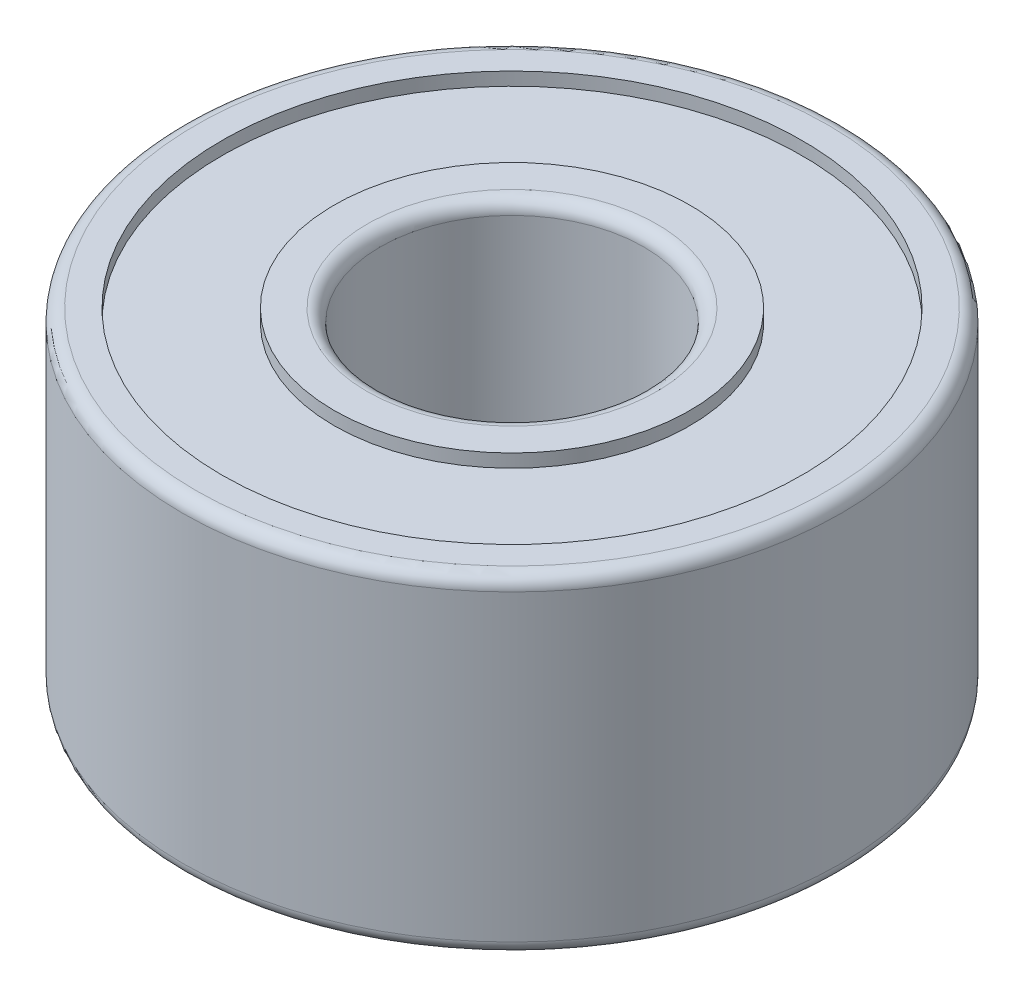
SolidWorks part; units mm, degrees
material "镀铬不锈钢"
ref_plane "前视基准面" through (0, 0, 0) normal (0, 0, 1) x (1, 0, 0)
ref_plane "上视基准面" through (0, 0, 0) normal (0, 1, 0) x (1, 0, 0)
ref_plane "右视基准面" through (0, 0, 0) normal (1, 0, 0) x (0, 0, -1)
sketch "草图1" plane through (0, 0, 0) normal (0, 1, 0) x (1, 0, 0)
  circle A0 centre (0, 0) radius 2.5
  circle A1 centre (0, 0) radius 1
  dimension "D1" = 5
  dimension "D2" = 2
extrude "凸台-拉伸1" add sketch "草图1" along normal blind 2.5
sketch "草图2" plane through (0, 2.5, 0) normal (0, 1, 0) x (1, 0, 0)
  circle A0 centre (0, 0) radius 2.2
  circle A1 centre (0, 0) radius 1.35
  dimension "D1" = 4.4
  dimension "D2" = 2.7
extrude "切除-拉伸1" cut sketch "草图2" against normal blind 0.1
sketch "草图4" plane through (0, 0, 0) normal (0, -1, 0) x (1, 0, 0)
  circle A1 centre (0, 0) radius 1.35
  circle A2 centre (0, 0) radius 1.35
  circle A3 centre (0, 0) radius 2.2
  circle A4 centre (0, 0) radius 2.2
  dimension "D1" = 0
  dimension "D2" = 0
extrude "切除-拉伸2" cut sketch "草图4" against normal blind 0.1
fillet "R0.1 圆角1" radius 0.1 4 edges at (0, 0, 1) (0, 0, 2.5) (0, 2.5, 1) (0, 2.5, 2.5)
